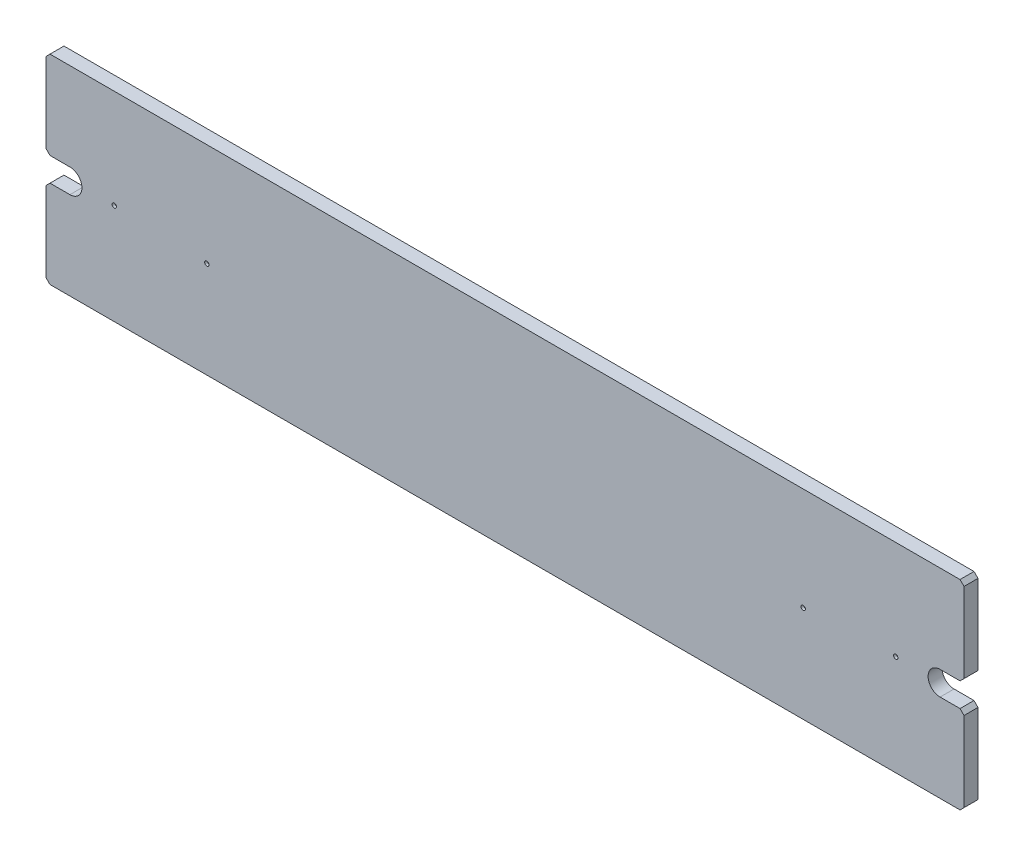
SolidWorks part; units mm, degrees
material "S45C"
ref_plane "Front Plane" through (0, 0, 0) normal (0, 0, 1) x (1, 0, 0)
ref_plane "Top Plane" through (0, 0, 0) normal (0, 1, 0) x (1, 0, 0)
ref_plane "Right Plane" through (0, 0, 0) normal (1, 0, 0) x (0, 0, -1)
sketch "Sketch1" plane through (0, 0, 0) normal (0, 0, 1) x (1, 0, 0)
  line L1 (-1150, 250) -> (1150, 250)
  line L2 (-1150, 250) -> (-1150, -250)
  line L3 (-1150, -250) -> (1150, -250)
  line L4 (1150, 250) -> (1150, -250)
  line L5 (-1150, 250) -> (1150, -250) construction
  line L6 (-1150, -250) -> (1150, 250) construction
  point P0 (0, 0)
  dimension "D1" = 2300
  dimension "D2" = 500
extrude "Boss-Extrude1" add sketch "Sketch1" along normal blind 35
sketch "Sketch2" plane through (0, 0, 0) normal (0, 0, -1) x (-1, 0, 0)
  circle A0 centre (-979, 2) radius 40
  circle A1 centre (979, 2) radius 40
  dimension "D1" = 80
extrude "Cut-Extrude1" cut sketch "Sketch2" against normal blind 5
sketch "Sketch3" plane through (0, 0, 0) normal (0, 0, -1) x (-1, 0, 0)
  line L0 (-947, -22) -> (-947, 26)
  line L1 (947, -22) -> (947, 26)
  line L2 (947, 22.4939) -> (947, -18.4939) construction
  line L3 (-947, -18.4939) -> (-947, 22.4939) construction
  arc A0 (-947, -22) -> (-947, 26) centre (-979, 2) ccw
  arc A1 (947, 26) -> (947, -22) centre (979, 2) ccw
  dimension "D1" = 80
extrude "Boss-Extrude2" add sketch "Sketch3" against normal blind 5
sketch "Sketch4" plane through (0, 0, 5) normal (0, 0, -1) x (-1, 0, 0)
  circle A0 centre (-947, -22) radius 2.5
  circle A1 centre (-947, 26) radius 2.5
  circle A2 centre (947, -22) radius 2.5
  circle A3 centre (947, 26) radius 2.5
  dimension "D1" = 5
extrude "Cut-Extrude2" cut sketch "Sketch4" against normal up to surface (5 mm away)
sketch "Sketch6" plane through (0, 0, 0) normal (0, 0, -1) x (-1, 0, 0)
  line L0 (-1150, 0) -> (1150, 0) construction
  line L1 (-1150, -250) -> (-1150, 250) construction
  line L2 (0, 0) -> (0, 250) construction
  line L3 (-1150, 250) -> (1150, 250) construction
  line L4 (1150, 250) -> (1150, -250) construction
  line L5 (1090, 0) -> (1190, 0) construction
  line L6 (1090, 30) -> (1190, 30)
  line L7 (1090, -30) -> (1190, -30)
  line L8 (-1090, 0) -> (-1190, 0) construction
  line L9 (-1090, 30) -> (-1190, 30)
  line L10 (-1090, -30) -> (-1190, -30)
  arc A0 (1090, 30) -> (1090, -30) centre (1090, 0) ccw
  arc A1 (1190, -30) -> (1190, 30) centre (1190, 0) ccw
  arc A2 (-1090, 30) -> (-1090, -30) centre (-1090, 0) cw
  arc A3 (-1190, -30) -> (-1190, 30) centre (-1190, 0) cw
  point P13 (1140, 0)
  point P21 (-1140, 0)
  dimension "D1" = 60
  dimension "D2" = 60
  dimension "D3" = 100
extrude "Cut-Extrude3" cut sketch "Sketch6" against normal through all
chamfer "Chamfer1" distance 10 angle 45 8 edges at (-1150, -30, 17.5) (-1150, 30, 17.5) (1150, -30, 17.5) (1150, 30, 17.5) (1150, 250, 17.5) (1150, -250, 17.5) (-1150, 250, 17.5) (-1150, -250, 17.5)
sketch "Sketch7" plane through (0, 0, 0) normal (0, 0, -1) x (-1, 0, 0)
  circle A0 centre (340, -76) radius 40
  circle A1 centre (397, 50) radius 40
  circle A2 centre (-2.98, 46) radius 40
  circle A3 centre (40, -76) radius 40
  circle A4 centre (-259.9583, -71) radius 40
  circle A5 centre (-397, 46) radius 40
  dimension "D1" = 80
extrude "Cut-Extrude4" cut sketch "Sketch7" against normal blind 5
hole_wizard "CBORE for M6 Hexagon socket head cap screws1" positions "Sketch9" profile "Sketch8" counterbore size "M6" standard "GB" end condition through all
sketch "Sketch9" plane through (0, 0, 35) normal (0, 0, 1) x (1, 0, 0)
  point P5 (-747, -8)
  point P23 (747, -8)
  point P27 (-979, 2)
  point P30 (979, 2)
sketch "Sketch8" plane through (-747, -8, 35) normal (1, 0, 0) x (0, -1, 0)
  line L0 (0, 0) -> (0, 35)
  line L1 (0, 35) -> (3.3, 35)
  line L3 (3.3, 35) -> (3.3, 6.8)
  line L4 (3.3, 6.8) -> (5.5, 6.8)
  line L5 (5.5, 6.8) -> (5.5, 0)
  line L7 (5.5, 0) -> (0, 0)
  line L11 (0, -6.35) -> (0, 107.95) construction
  dimension "通孔孔直径" = 6.6
  dimension "通孔孔深度" = 35
  dimension "柱形沉头孔直径" = 11
  dimension "柱形沉头孔深度" = 6.8
hole_wizard "M8 Tapped Hole1" positions "Sketch11" profile "Sketch10" tap size "M8" standard "GB"
sketch "Sketch11" plane through (0, 0, 0) normal (0, 0, -1) x (-1, 0, 0)
  circle A0 centre (735.5, -125) radius 4.5 construction
  circle A1 centre (595.5, -125) radius 4.5 construction
  circle A2 centre (735.5, 124) radius 4.5 construction
  circle A3 centre (595.5, 124) radius 4.5 construction
  circle A4 centre (-604.5, -125) radius 4.5 construction
  circle A5 centre (-744.5, -125) radius 4.5 construction
  circle A6 centre (-604.5, 124) radius 4.5 construction
  circle A7 centre (-744.5, 124) radius 4.5 construction
  point P1 (735.5, -125)
  point P5 (595.5, -125)
  point P9 (735.5, 124)
  point P13 (595.5, 124)
  point P17 (-604.5, -125)
  point P21 (-744.5, -125)
  point P25 (-604.5, 124)
  point P29 (-744.5, 124)
sketch "Sketch10" plane through (-735.5, -125, 0) normal (1, 0, 0) x (0, 1, 0)
  line L0 (0, 0) -> (0, 21.0429)
  line L1 (0, 21.0429) -> (3.4, 19)
  line L2 (3.4, 19) -> (3.4, 0)
  line L5 (3.4, 0) -> (0, 0)
  line L10 (0, 21.0429) -> (-3.4, 19) construction
  line L11 (0, -6.35) -> (0, 107.95) construction
  dimension "螺纹孔钻头直径" = 6.8
  dimension "螺纹孔钻头深度" = 19
  dimension "导头角度" = 118
cosmetic thread "Hole thread1" parameters "D1"=16, "D2"=8
cosmetic thread "Hole thread2" parameters "D1"=16, "D2"=8
cosmetic thread "Hole thread3" parameters "D1"=16, "D2"=8
cosmetic thread "Hole thread4" parameters "D1"=16, "D2"=8
cosmetic thread "Hole thread5" parameters "D1"=16, "D2"=8
cosmetic thread "Hole thread6" parameters "D1"=16, "D2"=8
cosmetic thread "Hole thread7" parameters "D1"=16, "D2"=8
cosmetic thread "Hole thread8" parameters "D1"=16, "D2"=8
